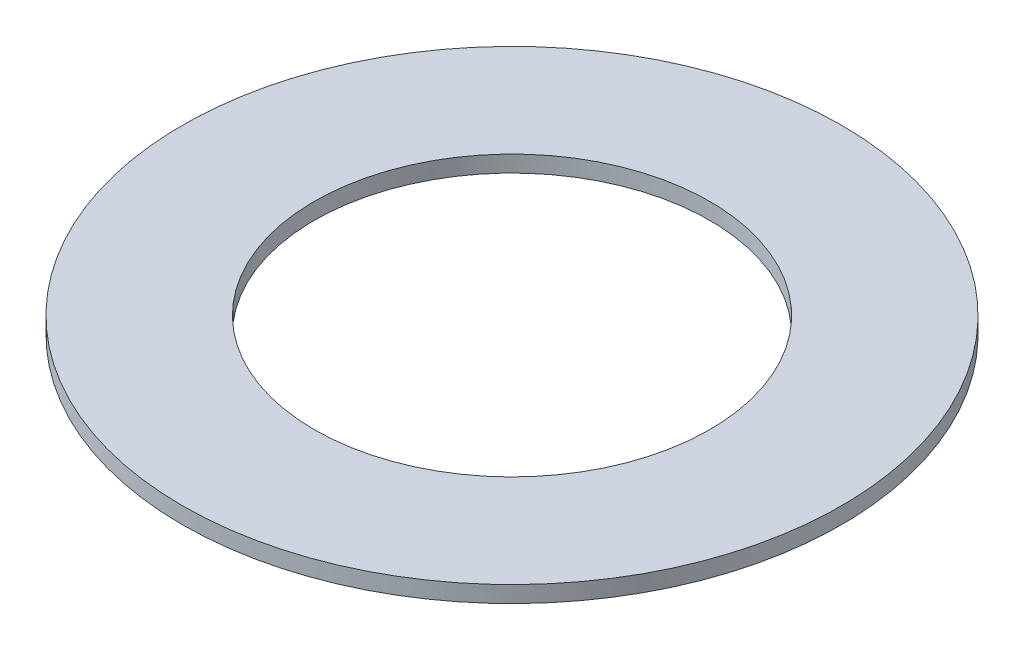
from build123d import *

# Parameters (mm, degrees)
SKETCH_1_R      = 10
SKETCH_1_R_2    = 6
EXTRUDE_1_DEPTH = 0.5


with BuildPart() as part:
    # 草图1 → 凸台-拉伸1 (new body)
    with BuildSketch(Plane(origin=(0, 0, 0), x_dir=(1, 0, 0), z_dir=(0, 1, 0))):
        with Locations(Location((0, 0, 0), (0, 0, 270))):
            Circle(SKETCH_1_R)
        with Locations(Location((0, 0, 0), (0, 0, 270))):
            Circle(SKETCH_1_R_2, mode=Mode.SUBTRACT)
    extrude(amount=EXTRUDE_1_DEPTH)


solid = part.part
